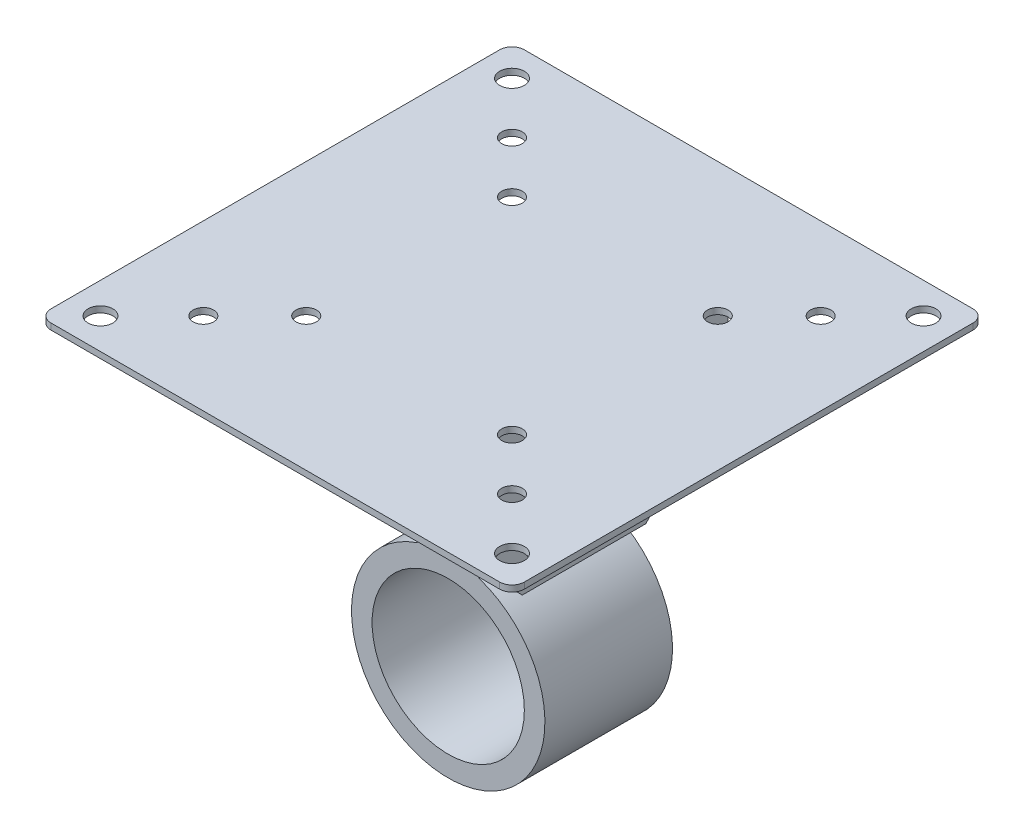
from build123d import *

# Parameters (mm, degrees)
SKETCH_1_W          = 115
SKETCH_1_H          = 115
EXTRUDE_1_DEPTH     = 0.75
SKETCH_2_R          = 2.5
CUT_EXTRUDE_1_DEPTH = 82.331113358
SKETCH_3_R          = 2.5
CUT_EXTRUDE_2_DEPTH = 82.331113358
SKETCH_4_R          = 3
CUT_EXTRUDE_3_DEPTH = 82.331113358
FILLET_1_R          = 3
SKETCH_5_W          = 35
SKETCH_5_H          = 70
EXTRUDE_2_DEPTH     = 41
CHAMFER_1_SIZE      = 20
SKETCH_6_R          = 18.5
EXTRUDE_3_DEPTH     = 15.5


with BuildPart() as part:
    # 草图1 → 凸台-拉伸1 (new, symmetric)
    with BuildSketch(Plane(origin=(0, 0, 0), x_dir=(1, 0, 0), z_dir=(0, 1, 0))):
        Rectangle(SKETCH_1_W, SKETCH_1_H)
    extrude(amount=EXTRUDE_1_DEPTH, both=True)

    # 草图2 → 切除-拉伸1 (cut, through all)
    with BuildSketch(Plane(origin=(0, 0.75, 0), x_dir=(1, 0, 0), z_dir=(0, 1, 0))):
        with Locations(Location((-25, 25, 0), (0, 0, 270))):
            Circle(SKETCH_2_R)
        with Locations(Location((25, 25, 0), (0, 0, 270))):
            Circle(SKETCH_2_R)
        with Locations(Location((25, -25, 0), (0, 0, 270))):
            Circle(SKETCH_2_R)
        with Locations(Location((-25, -25, 0), (0, 0, 270))):
            Circle(SKETCH_2_R)
    extrude(amount=-CUT_EXTRUDE_1_DEPTH, mode=Mode.SUBTRACT)

    # 草图3 → 切除-拉伸2 (cut, through all)
    with BuildSketch(Plane(origin=(0, 0.75, 0), x_dir=(1, 0, 0), z_dir=(0, 1, 0))):
        with Locations(Location((-37.5, 37.5, 0), (0, 0, 270))):
            Circle(SKETCH_3_R)
        with Locations(Location((-37.5, -37.5, 0), (0, 0, 270))):
            Circle(SKETCH_3_R)
        with Locations(Location((37.5, -37.5, 0), (0, 0, 270))):
            Circle(SKETCH_3_R)
        with Locations(Location((37.5, 37.5, 0), (0, 0, 270))):
            Circle(SKETCH_3_R)
    extrude(amount=-CUT_EXTRUDE_2_DEPTH, mode=Mode.SUBTRACT)

    # 草图4 → 切除-拉伸3 (cut, through all)
    with BuildSketch(Plane(origin=(0, 0.75, 0), x_dir=(1, 0, 0), z_dir=(0, 1, 0))):
        with Locations(Location((-50, 50, 0), (0, 0, 270))):
            Circle(SKETCH_4_R)
        with Locations(Location((50, 50, 0), (0, 0, 270))):
            Circle(SKETCH_4_R)
        with Locations(Location((-50, -50, 0), (0, 0, 270))):
            Circle(SKETCH_4_R)
        with Locations(Location((50, -50, 0), (0, 0, 270))):
            Circle(SKETCH_4_R)
    extrude(amount=-CUT_EXTRUDE_3_DEPTH, mode=Mode.SUBTRACT)

    # 圆角1
    fillet_1_edges = [part.edges().sort_by_distance(p)[0] for p in [
        (-57.5, 0, -57.5),
        (57.5, 0, -57.5),
        (57.5, 0, 57.5),
        (-57.5, 0, 57.5),
    ]]
    fillet(fillet_1_edges, radius=FILLET_1_R)

    # 草图5 → 凸台-拉伸2 (add)
    with BuildSketch(Plane.XZ.offset(0.75)):
        Rectangle(SKETCH_5_W, SKETCH_5_H)
    extrude(amount=EXTRUDE_2_DEPTH)

    # 倒角1
    chamfer_1_edges = [part.edges().sort_by_distance(p)[0] for p in [
        (0, -41.75, -35),
        (0, -41.75, 35),
    ]]
    chamfer(chamfer_1_edges, length=CHAMFER_1_SIZE)

    # 草图6 → 凸台-拉伸3 (add, symmetric)
    with BuildSketch(Plane.XY):
        with BuildLine():
            Line((7.5, -41.75), (7.5, -42.978942549))
            ThreePointArc((7.5, -42.978942549), (0, -88.75), (-7.5, -42.978942549))
            Line((-7.5, -42.978942549), (-7.5, -41.75))
            Line((-7.5, -41.75), (7.5, -41.75))
        make_face()
        with Locations((0, -65.25)):
            Circle(SKETCH_6_R, mode=Mode.SUBTRACT)
    extrude(amount=EXTRUDE_3_DEPTH, both=True)


solid = part.part
